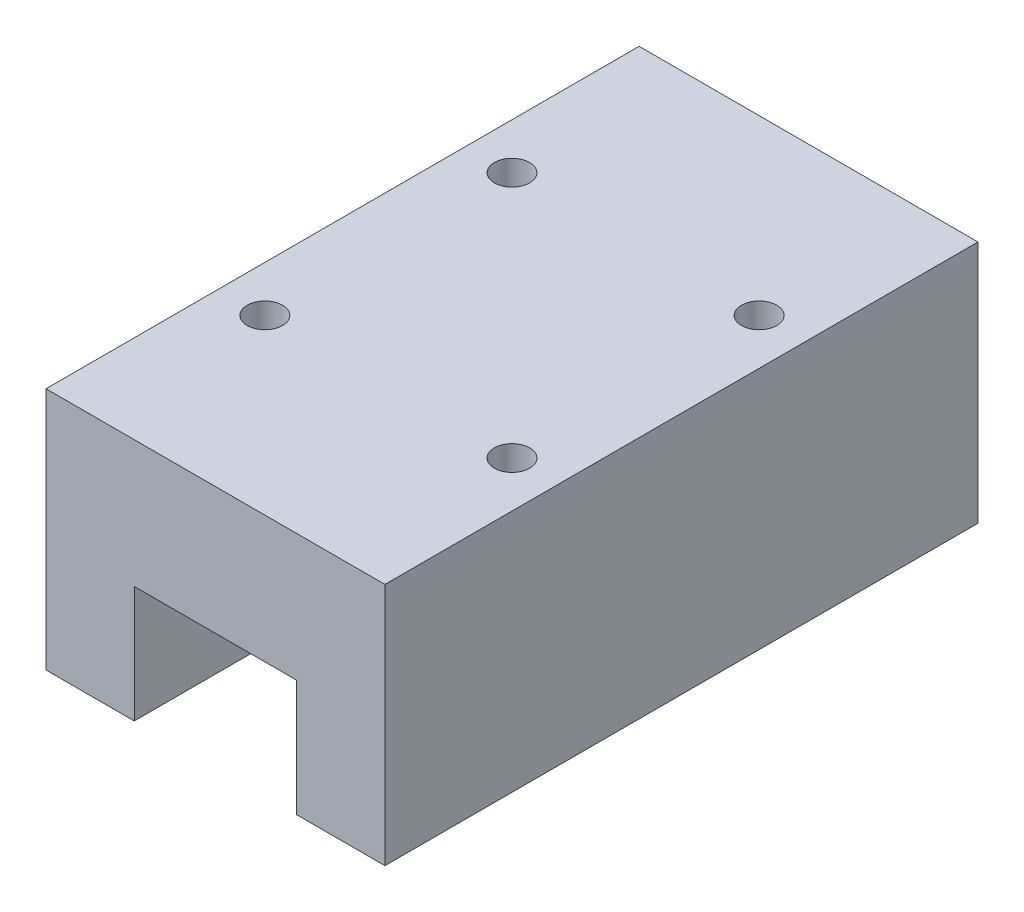
SolidWorks part; units mm, degrees
ref_plane "前视基准面" through (0, 0, 0) normal (0, 0, 1) x (1, 0, 0)
ref_plane "上视基准面" through (0, 0, 0) normal (0, 1, 0) x (1, 0, 0)
ref_plane "右视基准面" through (0, 0, 0) normal (1, 0, 0) x (0, 0, -1)
sketch "草图1" plane through (0, 0, 0) normal (0, 0, 1) x (1, 0, 0)
  line L0 (-11.5, -17.25) -> (-24, -17.25)
  line L1 (24, -17.25) -> (11.5, -17.25)
  line L2 (24, -17.25) -> (24, 17.25)
  line L3 (24, 17.25) -> (-24, 17.25)
  line L4 (-24, -17.25) -> (-24, 17.25)
  line L5 (24, -17.25) -> (-24, 17.25) construction
  line L6 (24, 17.25) -> (-24, -17.25) construction
  line L7 (-11.5, -0.75) -> (11.5, -0.75)
  line L8 (-11.5, -0.75) -> (-11.5, -17.25)
  line L10 (11.5, -0.75) -> (11.5, -17.25)
  point P0 (0, 0)
  dimension "D1" = 34.5
  dimension "D2" = 48
  dimension "D3" = 18
  dimension "D4" = 12.5
extrude "凸台-拉伸1" add sketch "草图1" along normal mid plane 84
hole_wizard "M6 螺纹孔1" positions "草图3" profile "草图2" tap size "M6" standard "GB"
sketch "草图3" plane through (0, 17.25, 0) normal (0, 1, 0) x (1, 0, 0)
  line L0 (-24, -42) -> (-24, 42) construction
  line L2 (24, -42) -> (-24, -42) construction
  point P0 (-17.5, 17.5)
  point P2 (17.5, 17.5)
  point P4 (17.5, -17.5)
  point P6 (-17.5, -17.5)
  dimension "D1" = 35
  dimension "D2" = 35
  dimension "D3" = 35
  dimension "D4" = 35
  dimension "D5" = 6.5
  dimension "D6" = 24.5
sketch "草图2" plane through (-17.5, 17.25, -17.5) normal (1, 0, 0) x (0, 0, 1)
  line L0 (0, 0) -> (0, 9.5022)
  line L1 (0, 9.5022) -> (2.5, 8)
  line L2 (2.5, 8) -> (2.5, 0)
  line L5 (2.5, 0) -> (0, 0)
  line L10 (0, 9.5022) -> (-2.5, 8) construction
  line L11 (0, -6.35) -> (0, 107.95) construction
  dimension "螺纹孔钻头直径" = 5
  dimension "螺纹孔钻头深度" = 8
  dimension "导头角度" = 118
cosmetic thread "孔螺蚊线1"
cosmetic thread "孔螺蚊线2"
cosmetic thread "孔螺蚊线3"
cosmetic thread "孔螺蚊线4"
